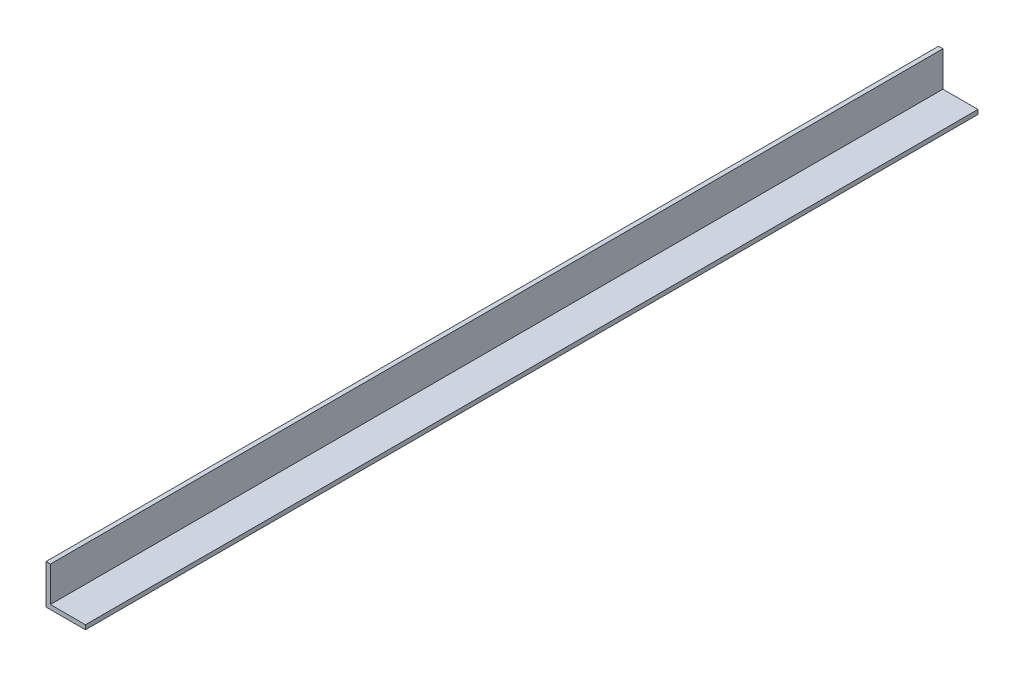
from build123d import *

# Parameters (mm, degrees)
EXTRUDE1_DEPTH = 1018.7


with BuildPart() as part:
    # Sketch1 → Extrude1 (new body)
    with BuildSketch(Plane.XY):
        Polygon((-46.706691722, 40), (-46.706691722, -5), (-1.706691722, -5), (-1.706691722, 0), (-41.706691722, 0), (-41.706691722, 40), align=None)
    extrude(amount=EXTRUDE1_DEPTH)


solid = part.part
